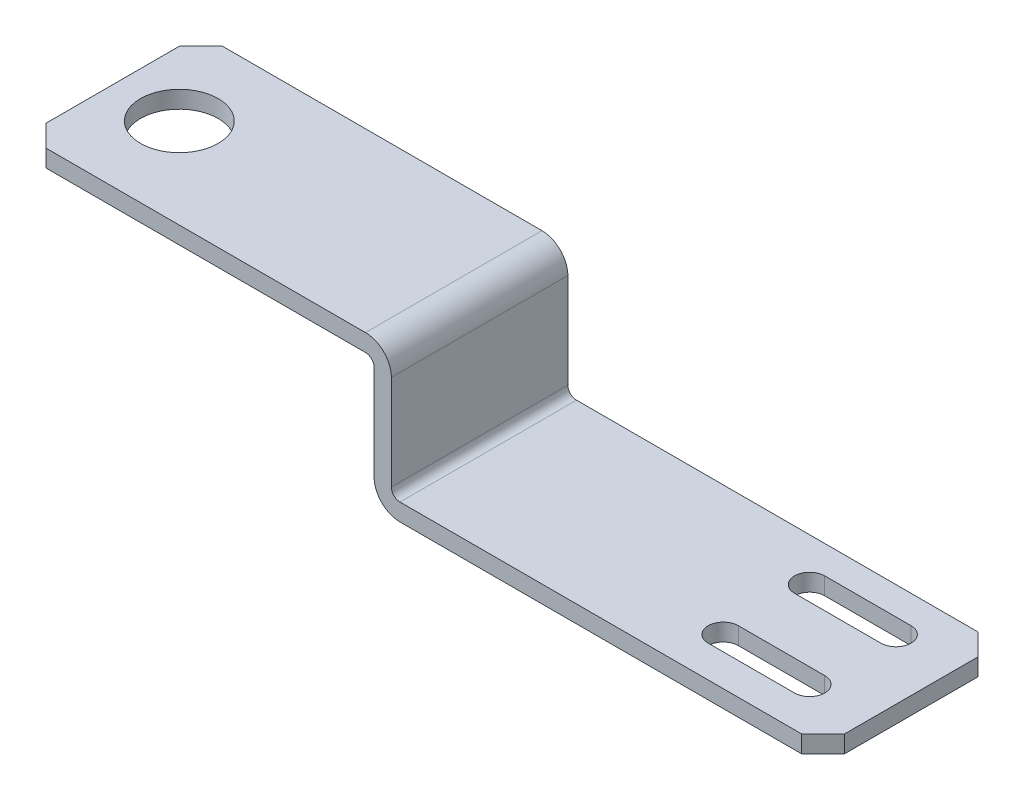
SolidWorks part; units mm, degrees
material "1023 碳钢板 (SS)"
ref_plane "前视基准面" through (0, 0, 0) normal (0, 0, 1) x (1, 0, 0)
ref_plane "上视基准面" through (0, 0, 0) normal (0, 1, 0) x (1, 0, 0)
ref_plane "右视基准面" through (0, 0, 0) normal (1, 0, 0) x (0, 0, -1)
ref_plane "基准面4" through (0, -30, 0) normal (0, -1, 0) x (1, 0, 0)
sketch "草图1" plane through (0, -30, 0) normal (0, -1, 0) x (1, 0, 0)
  line L0 (0, 0) -> (185, 0)
  line L1 (185, 0) -> (185, 40.884)
  line L2 (185, 40.884) -> (0, 40.884)
  line L3 (0, 40.884) -> (0, 0)
  dimension "D1" = 185
extrude "凸台-拉伸1" add sketch "草图1" against normal blind 34
sketch "草图2" plane through (0, 0, 0) normal (0, 0, -1) x (-1, 0, 0)
  line L0 (-185, -26) -> (-85, -26)
  line L1 (-85, -26) -> (-85, 4)
  line L2 (-85, 4) -> (-185, 4)
  line L3 (-185, 4) -> (-185, -26)
  line L4 (-185, 4) -> (-185, -30) construction
  dimension "D1" = 30
  dimension "D2" = 100
extrude "切除-拉伸1" cut sketch "草图2" against normal through all
sketch "草图3" plane through (0, 0, 0) normal (0, 0, -1) x (-1, 0, 0)
  line L0 (0, -30) -> (0, 0)
  line L1 (0, 0) -> (-81, 0)
  line L2 (-81, 0) -> (-81, -30)
  line L3 (-81, -30) -> (0, -30)
  dimension "D1" = 30
extrude "切除-拉伸2" cut sketch "草图3" against normal through all
sketch "草图4" plane through (0, -30, 0) normal (0, -1, 0) x (1, 0, 0)
  line L0 (171, 13.5) -> (151, 13.5)
  line L1 (151, 6.5) -> (171, 6.5)
  arc A0 (171, 6.5) -> (171, 13.5) centre (171, 10) ccw
  arc A1 (151, 13.5) -> (151, 6.5) centre (151, 10) ccw
extrude "切除-拉伸3" cut sketch "草图4" against normal through all
sketch "草图5" plane through (0, -26, 0) normal (0, 1, 0) x (-1, 0, 0)
  line L0 (-151, 33.5) -> (-171, 33.5)
  line L1 (-171, 26.5) -> (-151, 26.5)
  arc A0 (-171, 33.5) -> (-171, 26.5) centre (-171, 30) ccw
  arc A1 (-151, 26.5) -> (-151, 33.5) centre (-151, 30) ccw
extrude "切除-拉伸4" cut sketch "草图5" against normal through all
hole_wizard "Ø18.0 (18) 直径孔1" positions "草图7" profile "草图6" hole size "Ø18.0" standard "ANSI Metric"
sketch "草图7" plane through (0, 0, 0) normal (0, -1, 0) x (-1, 0, 0)
  point P0 (-15, -20)
sketch "草图6" plane through (15, 0, 20) normal (1, 0, 0) x (0, 0, -1)
  line L0 (0, 0) -> (0, 4)
  line L1 (0, 4) -> (9, 4)
  line L2 (9, 4) -> (9, 0)
  line L5 (9, 0) -> (0, 0)
  line L11 (0, -6.35) -> (0, 107.95) construction
  dimension "通孔孔直径" = 18
  dimension "通孔孔深度" = 4
chamfer "倒角1" distance 5 angle 45 4 edges at (0, 2, 40.884) (185, -28, 0) (0, 2, 0) (185, -28, 40.884)
fillet "圆角1" radius 2 2 edges at (85, -26, 20.442) (81, 0, 20.442)
fillet "圆角2" radius 6 2 edges at (81, -30, 20.442) (85, 4, 20.442)
